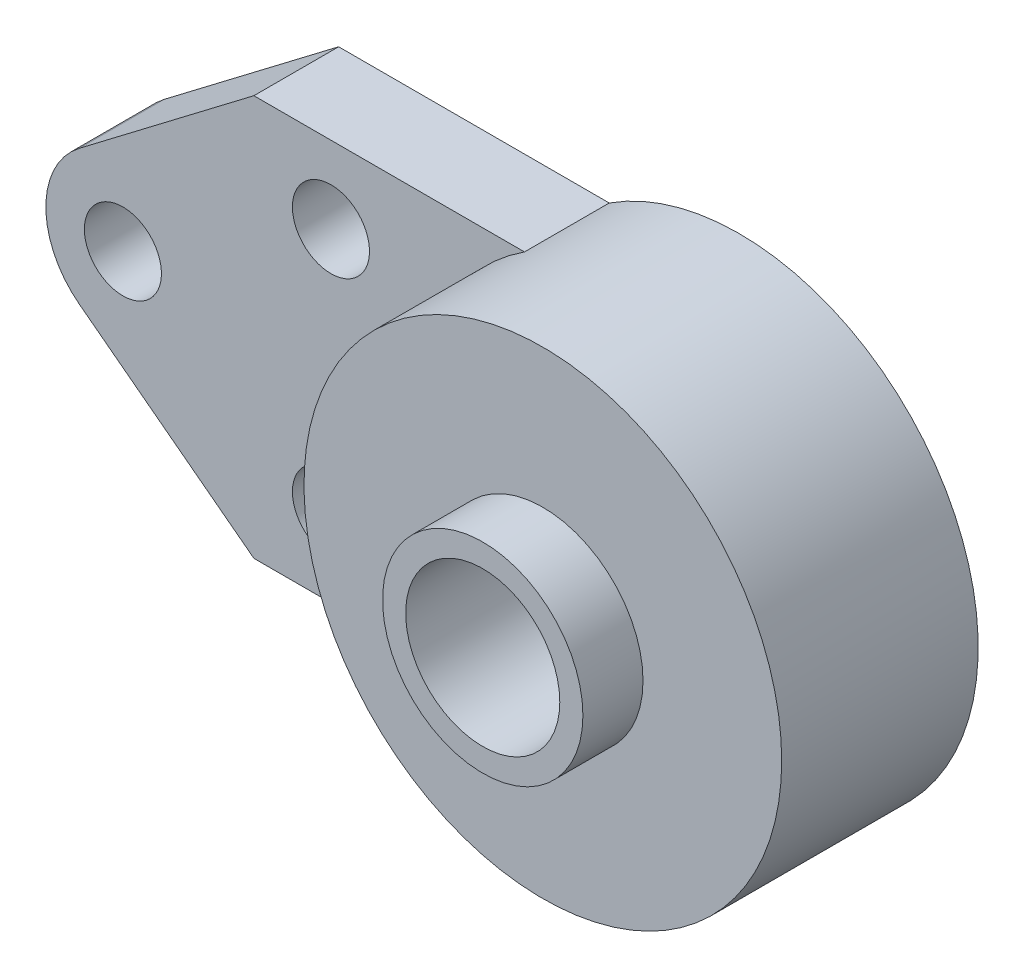
from build123d import *

# Parameters (mm, degrees)
SKETCH_1_R      = 31
SKETCH_1_R_2    = 10
EXTRUDE_1_DEPTH = 25.5
SKETCH_2_R      = 5
EXTRUDE_2_DEPTH = 11
SKETCH_3_R      = 13
SKETCH_3_R_2    = 10
EXTRUDE_3_DEPTH = 7.8


with BuildPart() as part:
    # 草图1 → 凸台-拉伸1 (new body)
    with BuildSketch(Plane.XY):
        Circle(SKETCH_1_R)
        Circle(SKETCH_1_R_2, mode=Mode.SUBTRACT)
    extrude(amount=EXTRUDE_1_DEPTH)

    # 草图2 → 凸台-拉伸2 (add)
    with BuildSketch(Plane(origin=(0, 0, 0), x_dir=(-1, 0, 0), z_dir=(0, 0, -1))):
        with BuildLine():
            Line((16.881943016, 26), (52, 26))
            Line((52, 26), (74.661722806, 8.753367881))
            ThreePointArc((74.661722806, 8.753367881), (79, 0), (74.661722806, -8.753367881))
            Line((74.661722806, -8.753367881), (52, -26))
            Line((52, -26), (16.881943016, -26))
            ThreePointArc((16.881943016, -26), (31, 0), (16.881943016, 26))
        make_face()
        with Locations((69, 0)):
            Circle(SKETCH_2_R, mode=Mode.SUBTRACT)
        with Locations((42, 16)):
            Circle(SKETCH_2_R, mode=Mode.SUBTRACT)
        with Locations((42, -16)):
            Circle(SKETCH_2_R, mode=Mode.SUBTRACT)
    extrude(amount=-EXTRUDE_2_DEPTH)

    # 草图3 → 凸台-拉伸3 (add)
    with BuildSketch(Plane.XY.offset(25.5)):
        Circle(SKETCH_3_R)
        Circle(SKETCH_3_R_2, mode=Mode.SUBTRACT)
    extrude(amount=EXTRUDE_3_DEPTH)


solid = part.part
